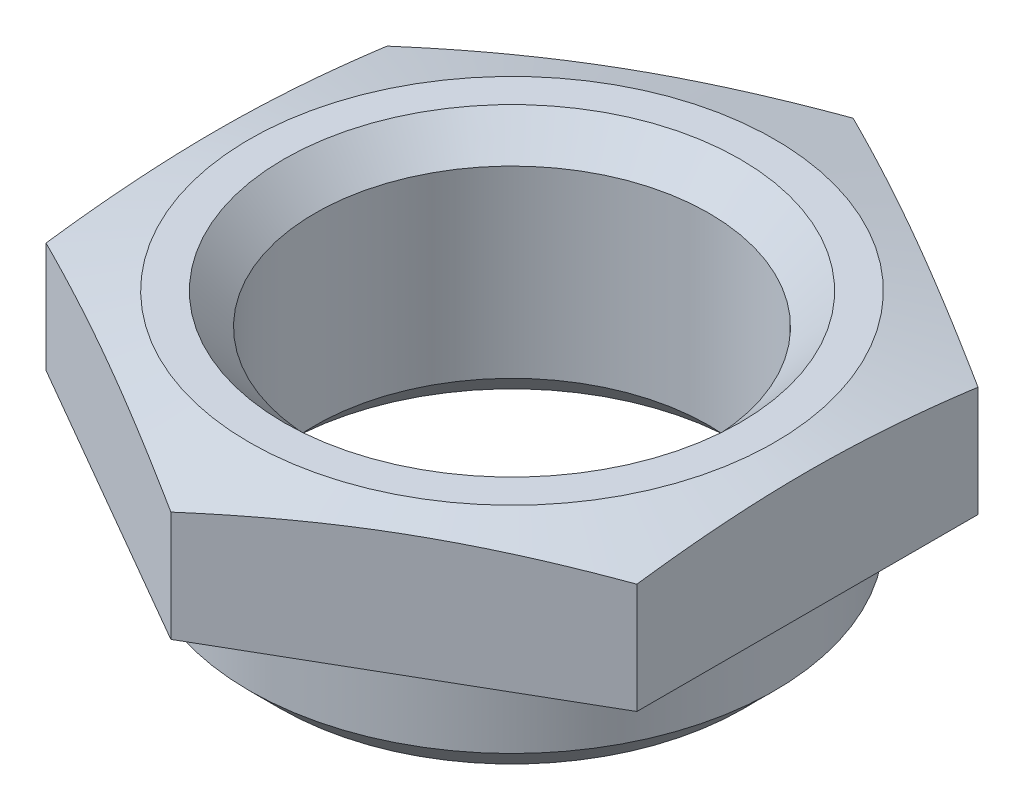
from build123d import *

# Parameters (mm, degrees)
EXTRUDE_1_DEPTH = 8


with BuildPart() as part:
    # 草图1 → 旋转1 (revolve)
    with BuildSketch(Plane.XY, mode=Mode.PRIVATE) as revolve_1_sk:
        Polygon((-13.9, 0), (-14.1, 0), (-16, 1.9), (-16, 7), (-18, 7), (-18, 14.464101615), (-16, 15), (-13.9, 15), (-12, 13.1), (-12, 1.9), align=None)
    revolve(revolve_1_sk.sketch.rotate(Axis((0, 0, 0), (0, -1, 0)), 270), axis=Axis((0, 0, 0), (0, -1, 0)))

    # 草图2 → 拉伸1 (add)
    with BuildSketch(Plane(origin=(0, 15, 0), x_dir=(1, 0, 0), z_dir=(0, 1, 0))):
        Polygon((18, -10.392304845), (18, 10.392304845), (0, 20.784609691), (-18, 10.392304845), (-18, -10.392304845), (0, -20.784609691), align=None)
    extrude(amount=-EXTRUDE_1_DEPTH)

    # 草图3 → 切除-旋转2 (revolve, cut)
    with BuildSketch(Plane.XY, mode=Mode.PRIVATE) as cut_revolve_2_sk:
        Polygon((-29.9, 11.275506225), (-16, 15), (-29.9, 15), align=None)
        Polygon((-13.9, 15), (-12, 13.1), (-12, 0), (0, 0), (0, 15), align=None)
    revolve(cut_revolve_2_sk.sketch.rotate(Axis((0, 0, 0), (0, -1, 0)), 270), axis=Axis((0, 0, 0), (0, -1, 0)), mode=Mode.SUBTRACT)


solid = part.part
